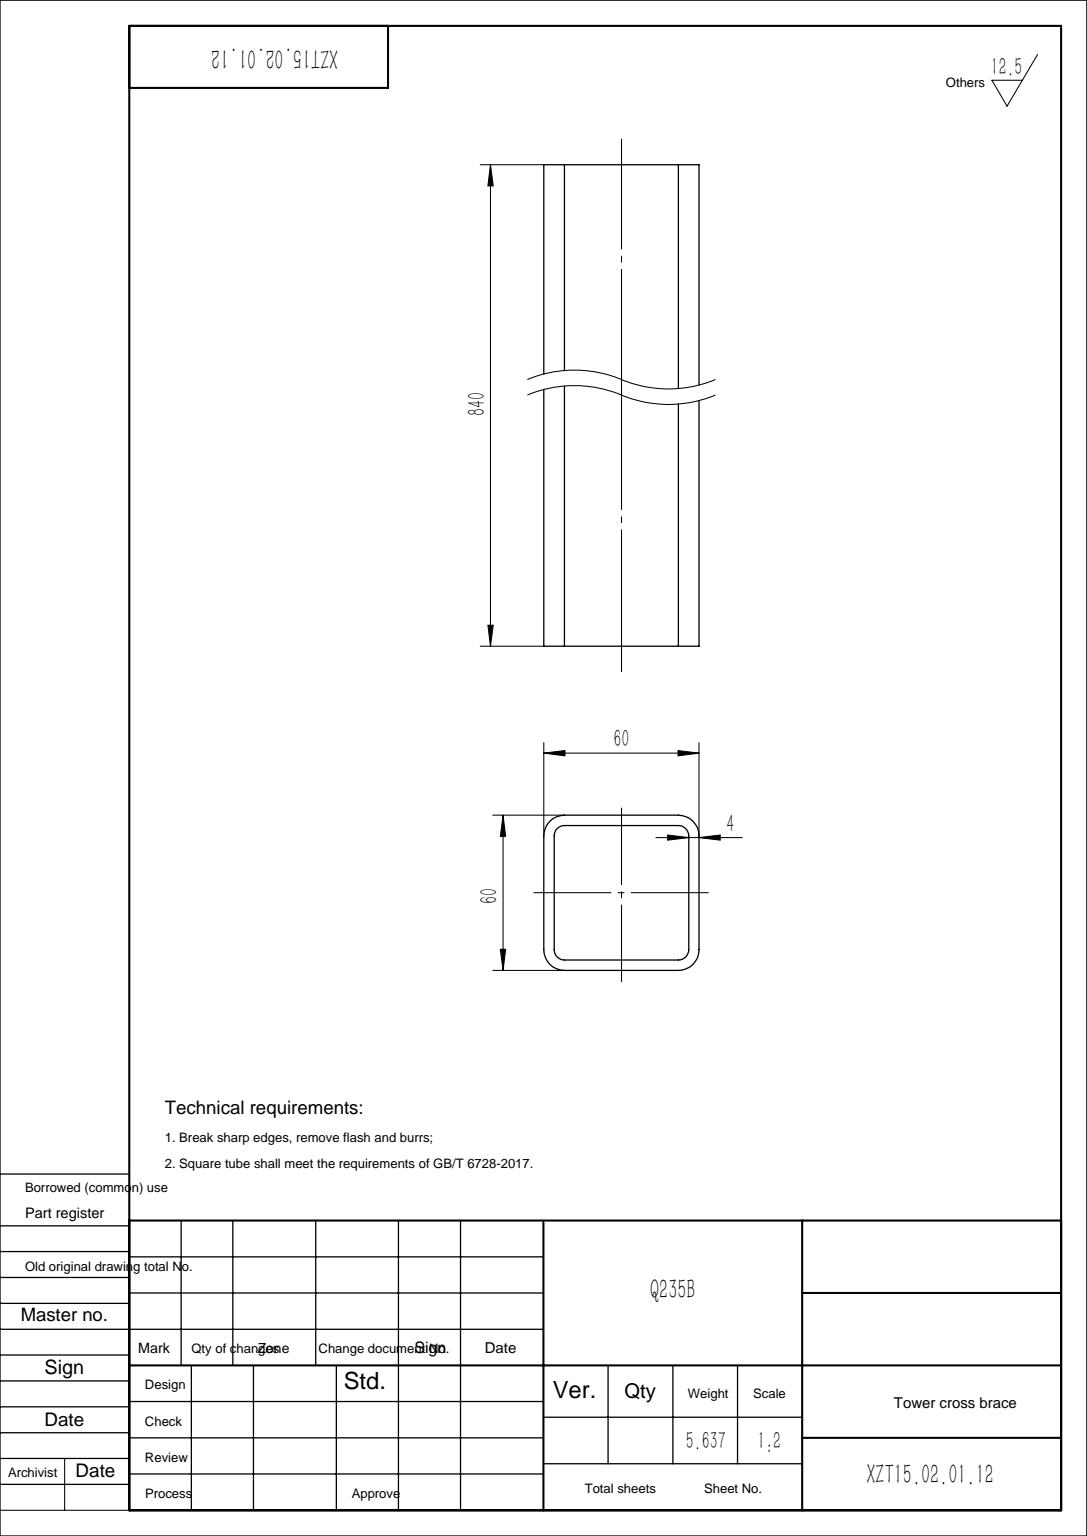
from build123d import *

# Parameters (mm, degrees)
GB_T_6728_2002_SQUARE_HOLLOW_SECTION_60_DEPTH = 840


with BuildPart() as part:
    # Sketch1 → GB/T 6728-2002 square hollow section 60×60×4(1) (new body)
    with BuildSketch(Plane(origin=(0, 0, 0), x_dir=(-1, 0, 0), z_dir=(0, 1, 0))):
        with BuildLine():
            Line((-22, -30), (22, -30))
            ThreePointArc((22, -30), (27.656854249, -27.656854249), (30, -22))
            Line((30, -22), (30, 22))
            ThreePointArc((30, 22), (27.656854249, 27.656854249), (22, 30))
            Line((22, 30), (-22, 30))
            ThreePointArc((-22, 30), (-27.656854249, 27.656854249), (-30, 22))
            Line((-30, 22), (-30, -22))
            ThreePointArc((-30, -22), (-27.656854249, -27.656854249), (-22, -30))
        make_face()
        with BuildLine():
            Line((-22, -26), (22, -26))
            ThreePointArc((22, -26), (24.828427125, -24.828427125), (26, -22))
            Line((26, -22), (26, 22))
            ThreePointArc((26, 22), (24.828427125, 24.828427125), (22, 26))
            Line((22, 26), (-22, 26))
            ThreePointArc((-22, 26), (-24.828427125, 24.828427125), (-26, 22))
            Line((-26, 22), (-26, -22))
            ThreePointArc((-26, -22), (-24.828427125, -24.828427125), (-22, -26))
        make_face(mode=Mode.SUBTRACT)
    extrude(amount=GB_T_6728_2002_SQUARE_HOLLOW_SECTION_60_DEPTH)


solid = part.part
